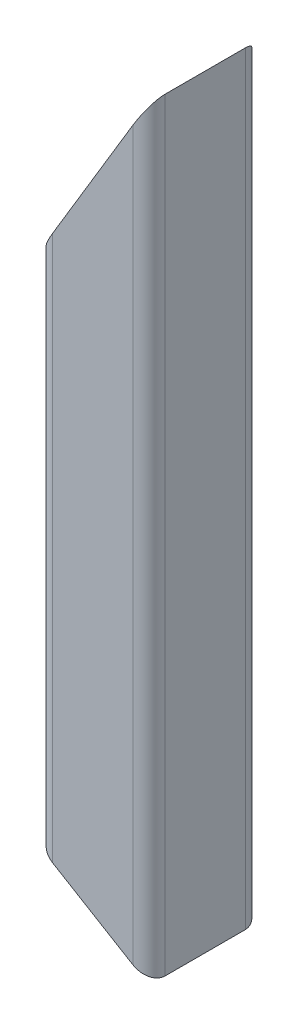
SolidWorks part; units mm, degrees
material "XRAAT"
ref_plane "前视基准面" through (0, 0, 0) normal (0, 0, 1) x (1, 0, 0)
ref_plane "上视基准面" through (0, 0, 0) normal (0, 1, 0) x (1, 0, 0)
ref_plane "右视基准面" through (0, 0, 0) normal (1, 0, 0) x (0, 0, -1)
sketch "草图1" plane through (0, 0, 0) normal (0, 0, 1) x (1, 0, 0)
  line L0 (0, 0) -> (0, 476)
  dimension "D1" = 476
other "结构用冷弯空心方钢(gb t6728-2002) 70×70×5(1)"
ref_plane "基准面1" through (0, 0, 0) normal (0, 1, 0) x (-1, 0, 0)
sketch "Sketch1" plane through (0, 0, 0) normal (0, 1, 0) x (-1, 0, 0)
  line L0 (-25, -30) -> (25, -30)
  line L1 (-30, -25) -> (-30, 25)
  line L2 (25, 30) -> (-25, 30)
  line L3 (30, 25) -> (30, -25)
  line L4 (-25, -35) -> (25, -35)
  line L5 (-35, -25) -> (-35, 25)
  line L6 (25, 35) -> (-25, 35)
  line L7 (35, 25) -> (35, -25)
  arc A0 (35, 25) -> (25, 35) centre (25, 25) ccw
  arc A1 (25, -35) -> (35, -25) centre (25, -25) ccw
  arc A2 (-35, -25) -> (-25, -35) centre (-25, -25) ccw
  arc A3 (-25, 35) -> (-35, 25) centre (-25, 25) ccw
  arc A4 (-25, 30) -> (-30, 25) centre (-25, 25) ccw
  arc A5 (30, 25) -> (25, 30) centre (25, 25) ccw
  arc A6 (25, -30) -> (30, -25) centre (25, -25) ccw
  arc A7 (-30, -25) -> (-25, -30) centre (-25, -25) ccw
  point P0 (-35, 0)
  point P1 (35, 0)
  point P2 (0, 35)
  point P3 (0, -35)
  point P4 (0, 0)
  point P5 (-35, -35)
  point P6 (35, -35)
  point P7 (35, 35)
  point P8 (-35, 35)
  point P33 (0, 0)
  dimension "D1" = 10
  dimension "D2" = 70
  dimension "D3" = 5
sketch "草图2" plane through (0, 0, 35) normal (0, 0, 1) x (1, 0, 0)
  line L0 (35, 476) -> (-35, 359.3333)
  line L1 (-35, 476) -> (-35, 0) construction
  line L2 (-35, 359.3333) -> (-35, 476)
  line L3 (-35, 476) -> (35, 476)
  line L4 (-35, 42) -> (35, 0)
  line L5 (35, 0) -> (-35, 0)
  line L6 (-35, 0) -> (-35, 42)
  dimension "D1" = 42
  dimension "D2" = 90
extrude "切除-拉伸1" cut sketch "草图2" against normal through all both and the other way through all
